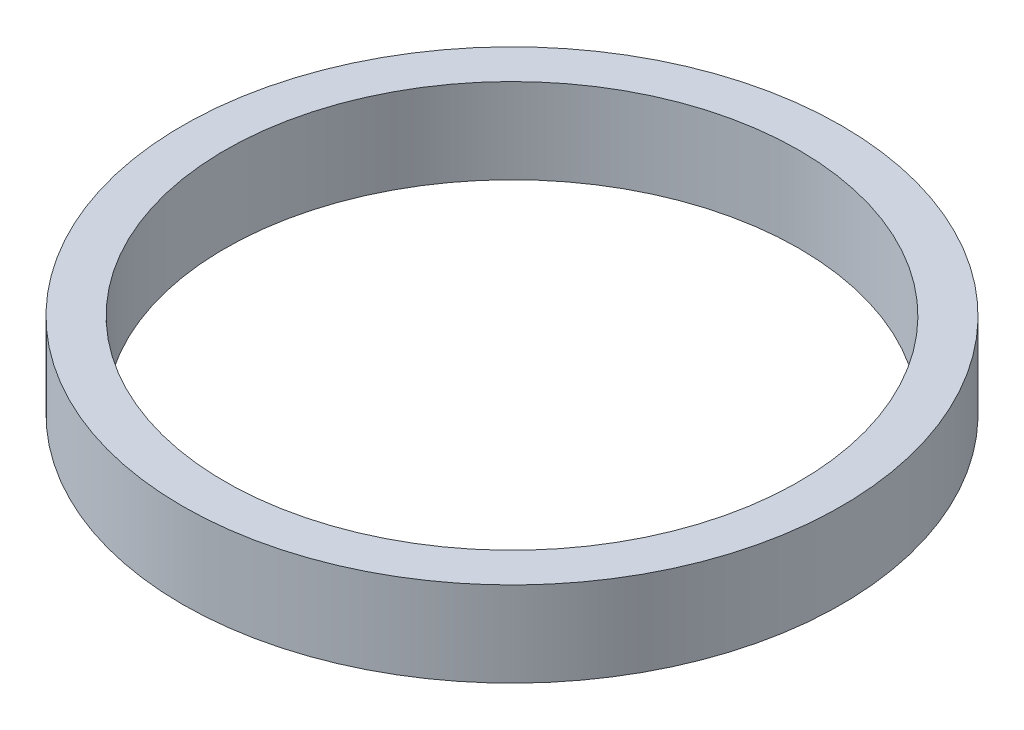
SolidWorks part; units mm, degrees
ref_plane "Front Plane" through (0, 0, 0) normal (0, 0, 1) x (1, 0, 0)
ref_plane "Top Plane" through (0, 0, 0) normal (0, 1, 0) x (1, 0, 0)
ref_plane "Right Plane" through (0, 0, 0) normal (1, 0, 0) x (0, 0, -1)
other "Configuration Table"
sketch "Sketch2" plane through (0, 0, 0) normal (0, 0, 1) x (1, 0, 0)
  line L0 (0, -1.5407) -> (0, 2.2476) construction
  line L1 (13.5, 0) -> (13.5, 4)
  line L3 (15.5, 4) -> (15.5, 0)
  line L4 (15.5, 0) -> (13.5, 0)
  line L5 (-3.1754, 0) -> (13.5, 0) construction
  line L10 (13.5, 0) -> (1015.2672, 0) construction
  line L15 (13.5, 4) -> (15.5, 4)
  dimension "D1" = 4
  dimension "D2" = 2
  dimension "D3" = 31
revolve "Revolve1" add sketch "Sketch2" angle 360 about L0
